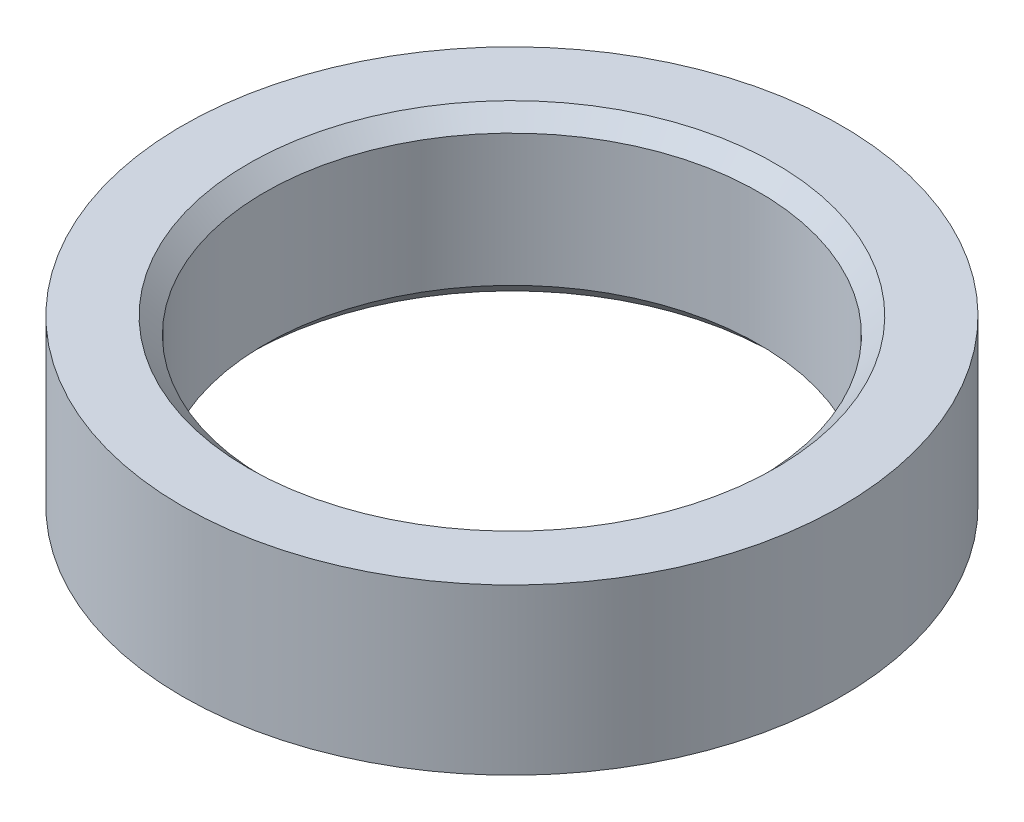
SolidWorks part; units mm, degrees
material "AISI 304"
ref_plane "前视基准面" through (0, 0, 0) normal (0, 0, 1) x (1, 0, 0)
ref_plane "上视基准面" through (0, 0, 0) normal (0, 1, 0) x (1, 0, 0)
ref_plane "右视基准面" through (0, 0, 0) normal (1, 0, 0) x (0, 0, -1)
sketch "草图1" plane through (0, 0, 0) normal (0, 1, 0) x (1, 0, 0)
  circle A0 centre (0, 0) radius 4
  circle A1 centre (0, 0) radius 3
  dimension "D1" = 8
  dimension "D2" = 6
extrude "凸台-拉伸1" add sketch "草图1" along normal blind 2
chamfer "C0.2 倒角1" distance 0.2 angle 45 2 edges at (0, 0, 3) (0, 2, 3)
